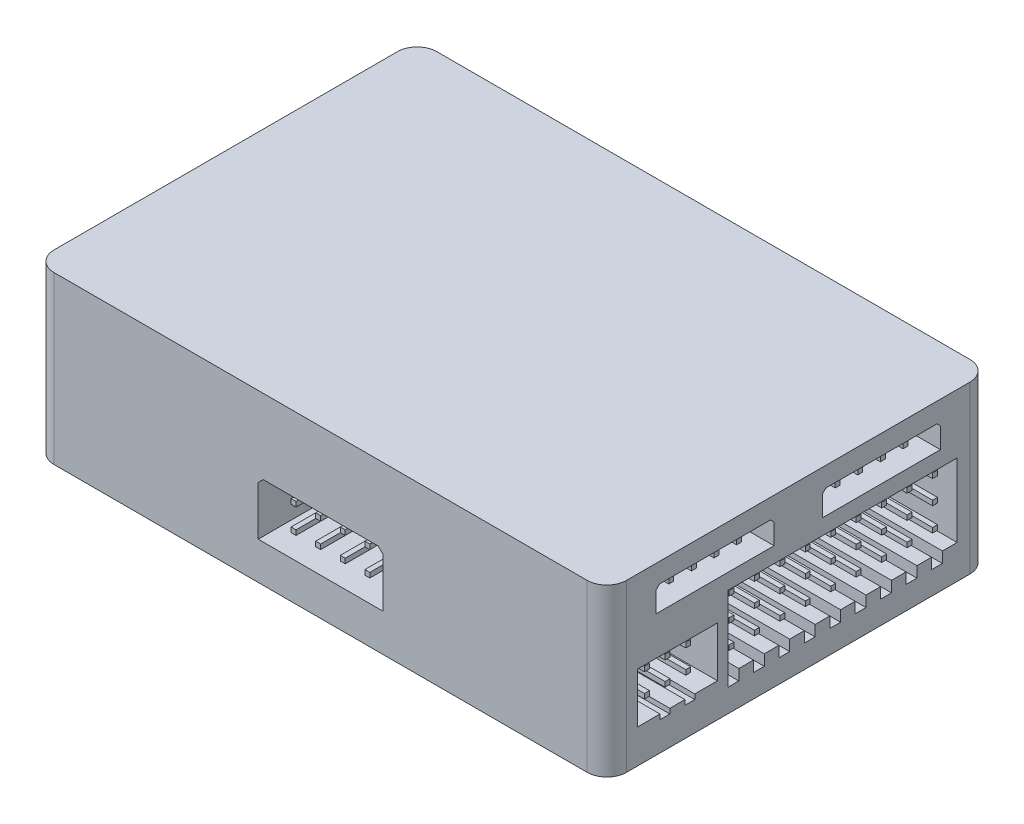
SolidWorks part; units mm, degrees
material "1060 合金"
ref_plane "前视基准面" through (0, 0, 0) normal (0, 0, 1) x (1, 0, 0)
ref_plane "上视基准面" through (0, 0, 0) normal (0, 1, 0) x (1, 0, 0)
ref_plane "右视基准面" through (0, 0, 0) normal (1, 0, 0) x (0, 0, -1)
other "质心 (COM)"
ref_plane "基准面4" through (0, 16.91, 0) normal (0, 1, 0) x (1, 0, 0)
sketch "草图1" plane through (0, 16.91, 0) normal (0, 1, 0) x (1, 0, 0)
  line L0 (29.105, -19.46) -> (29.105, 19.46)
  line L1 (29.105, 19.46) -> (-29.105, 19.46)
  line L2 (-29.105, 19.46) -> (-29.105, -19.46)
  line L3 (-29.105, -19.46) -> (29.105, -19.46)
extrude "凸台-拉伸1" add sketch "草图1" against normal blind 16.91
sketch "草图2" plane through (0, 0, 19.46) normal (0, 0, 1) x (1, 0, 0)
  line L0 (-6.35, 3.81) -> (6.35, 3.81)
  line L1 (6.35, 3.81) -> (6.35, 9.31)
  line L2 (6.35, 9.31) -> (-6.35, 9.31)
  line L3 (-6.35, 9.31) -> (-6.35, 3.81)
extrude "切除-拉伸1" cut sketch "草图2" against normal blind 10
sketch "草图3" plane through (0, 0, 9.46) normal (0, 0, 1) x (1, 0, 0)
  line L0 (-4, 8.06) -> (-3.5, 8.06)
  line L1 (-3.5, 8.06) -> (-3.5, 7.56)
  line L2 (-3.5, 7.56) -> (-4, 7.56)
  line L3 (-4, 7.56) -> (-4, 8.06)
extrude "凸台-拉伸2" add sketch "草图3" along normal blind 9
sketch "草图4" plane through (0, 0, 9.46) normal (0, 0, 1) x (1, 0, 0)
  line L0 (-4, 5.56) -> (-3.5, 5.56)
  line L1 (-3.5, 5.56) -> (-3.5, 5.06)
  line L2 (-3.5, 5.06) -> (-4, 5.06)
  line L3 (-4, 5.06) -> (-4, 5.56)
extrude "凸台-拉伸3" add sketch "草图4" along normal blind 9
sketch "草图5" plane through (0, 0, 9.46) normal (0, 0, 1) x (1, 0, 0)
  line L0 (-1.5, 8.06) -> (-1, 8.06)
  line L1 (-1, 8.06) -> (-1, 7.56)
  line L2 (-1, 7.56) -> (-1.5, 7.56)
  line L3 (-1.5, 7.56) -> (-1.5, 8.06)
extrude "凸台-拉伸4" add sketch "草图5" along normal blind 9
sketch "草图6" plane through (0, 0, 9.46) normal (0, 0, 1) x (1, 0, 0)
  line L0 (-1.5, 5.56) -> (-1, 5.56)
  line L1 (-1, 5.56) -> (-1, 5.06)
  line L2 (-1, 5.06) -> (-1.5, 5.06)
  line L3 (-1.5, 5.06) -> (-1.5, 5.56)
extrude "凸台-拉伸5" add sketch "草图6" along normal blind 9
sketch "草图7" plane through (0, 0, 9.46) normal (0, 0, 1) x (1, 0, 0)
  line L0 (1.5, 5.56) -> (1.5, 5.06)
  line L1 (1.5, 5.06) -> (1, 5.06)
  line L2 (1, 5.06) -> (1, 5.56)
  line L3 (1, 5.56) -> (1.5, 5.56)
extrude "凸台-拉伸6" add sketch "草图7" along normal blind 9
sketch "草图8" plane through (0, 0, 9.46) normal (0, 0, 1) x (1, 0, 0)
  line L0 (1.5, 8.06) -> (1.5, 7.56)
  line L1 (1.5, 7.56) -> (1, 7.56)
  line L2 (1, 7.56) -> (1, 8.06)
  line L3 (1, 8.06) -> (1.5, 8.06)
extrude "凸台-拉伸7" add sketch "草图8" along normal blind 9
sketch "草图9" plane through (0, 0, 9.46) normal (0, 0, 1) x (1, 0, 0)
  line L0 (4, 5.56) -> (4, 5.06)
  line L1 (4, 5.06) -> (3.5, 5.06)
  line L2 (3.5, 5.06) -> (3.5, 5.56)
  line L3 (3.5, 5.56) -> (4, 5.56)
extrude "凸台-拉伸8" add sketch "草图9" along normal blind 9
sketch "草图10" plane through (0, 0, 9.46) normal (0, 0, 1) x (1, 0, 0)
  line L0 (4, 8.06) -> (4, 7.56)
  line L1 (4, 7.56) -> (3.5, 7.56)
  line L2 (3.5, 7.56) -> (3.5, 8.06)
  line L3 (3.5, 8.06) -> (4, 8.06)
extrude "凸台-拉伸9" add sketch "草图10" along normal blind 9
sketch "草图11" plane through (29.105, 0, 0) normal (1, 0, 0) x (0, 0, -1)
  line L0 (13.56, 2.34) -> (14.66, 2.34)
  line L1 (14.66, 2.34) -> (14.66, 3.44)
  line L2 (14.66, 3.44) -> (16.16, 3.44)
  line L3 (16.16, 3.44) -> (16.16, 10.88)
  line L4 (16.16, 10.88) -> (-7.14, 10.88)
  line L5 (-7.14, 10.88) -> (-7.14, 2.34)
  line L6 (-7.14, 2.34) -> (-6.04, 2.34)
  line L7 (-6.04, 2.34) -> (-6.04, 3.44)
  line L8 (-6.04, 3.44) -> (-4.5525, 3.44)
  line L9 (-4.5525, 3.44) -> (-4.5525, 2.34)
  line L10 (-4.5525, 2.34) -> (-3.4525, 2.34)
  line L11 (-3.4525, 2.34) -> (-3.4525, 3.44)
  line L12 (-3.4525, 3.44) -> (-1.965, 3.44)
  line L13 (-1.965, 3.44) -> (-1.965, 2.34)
  line L14 (-1.965, 2.34) -> (-0.865, 2.34)
  line L15 (-0.865, 2.34) -> (-0.865, 3.44)
  line L16 (-0.865, 3.44) -> (0.6225, 3.44)
  line L17 (0.6225, 3.44) -> (0.6225, 2.34)
  line L18 (0.6225, 2.34) -> (1.7225, 2.34)
  line L19 (1.7225, 2.34) -> (1.7225, 3.44)
  line L20 (1.7225, 3.44) -> (3.21, 3.44)
  line L21 (3.21, 3.44) -> (3.21, 2.34)
  line L22 (3.21, 2.34) -> (4.31, 2.34)
  line L23 (4.31, 2.34) -> (4.31, 3.44)
  line L24 (4.31, 3.44) -> (5.7975, 3.44)
  line L25 (5.7975, 3.44) -> (5.7975, 2.34)
  line L26 (5.7975, 2.34) -> (6.8975, 2.34)
  line L27 (6.8975, 2.34) -> (6.8975, 3.44)
  line L28 (6.8975, 3.44) -> (8.385, 3.44)
  line L29 (8.385, 3.44) -> (8.385, 2.34)
  line L30 (8.385, 2.34) -> (9.485, 2.34)
  line L31 (9.485, 2.34) -> (9.485, 3.44)
  line L32 (9.485, 3.44) -> (10.9725, 3.44)
  line L33 (10.9725, 3.44) -> (10.9725, 2.34)
  line L34 (10.9725, 2.34) -> (12.0725, 2.34)
  line L35 (12.0725, 2.34) -> (12.0725, 3.44)
  line L36 (12.0725, 3.44) -> (13.56, 3.44)
  line L37 (13.56, 3.44) -> (13.56, 2.34)
extrude "切除-拉伸2" cut sketch "草图11" against normal blind 10
sketch "草图12" plane through (19.105, 0, 0) normal (1, 0, 0) x (0, 0, -1)
  line L0 (14.66, 7.41) -> (15.16, 7.41)
  line L1 (15.16, 7.41) -> (15.16, 6.91)
  line L2 (15.16, 6.91) -> (14.66, 6.91)
  line L3 (14.66, 6.91) -> (14.66, 7.41)
extrude "凸台-拉伸10" add sketch "草图12" along normal blind 9
sketch "草图13" plane through (19.105, 0, 0) normal (1, 0, 0) x (0, 0, -1)
  line L0 (12.0725, 5.01) -> (12.5725, 5.01)
  line L1 (12.5725, 5.01) -> (12.5725, 4.51)
  line L2 (12.5725, 4.51) -> (12.0725, 4.51)
  line L3 (12.0725, 4.51) -> (12.0725, 5.01)
extrude "凸台-拉伸11" add sketch "草图13" along normal blind 9
sketch "草图14" plane through (19.105, 0, 0) normal (1, 0, 0) x (0, 0, -1)
  line L0 (12.0725, 9.81) -> (12.5725, 9.81)
  line L1 (12.5725, 9.81) -> (12.5725, 9.31)
  line L2 (12.5725, 9.31) -> (12.0725, 9.31)
  line L3 (12.0725, 9.31) -> (12.0725, 9.81)
extrude "凸台-拉伸12" add sketch "草图14" along normal blind 9
sketch "草图15" plane through (19.105, 0, 0) normal (1, 0, 0) x (0, 0, -1)
  line L0 (9.485, 7.41) -> (9.985, 7.41)
  line L1 (9.985, 7.41) -> (9.985, 6.91)
  line L2 (9.985, 6.91) -> (9.485, 6.91)
  line L3 (9.485, 6.91) -> (9.485, 7.41)
extrude "凸台-拉伸13" add sketch "草图15" along normal blind 9
sketch "草图16" plane through (19.105, 0, 0) normal (1, 0, 0) x (0, 0, -1)
  line L0 (6.8975, 5.01) -> (7.3975, 5.01)
  line L1 (7.3975, 5.01) -> (7.3975, 4.51)
  line L2 (7.3975, 4.51) -> (6.8975, 4.51)
  line L3 (6.8975, 4.51) -> (6.8975, 5.01)
extrude "凸台-拉伸14" add sketch "草图16" along normal blind 9
sketch "草图17" plane through (19.105, 0, 0) normal (1, 0, 0) x (0, 0, -1)
  line L0 (6.8975, 9.81) -> (7.3975, 9.81)
  line L1 (7.3975, 9.81) -> (7.3975, 9.31)
  line L2 (7.3975, 9.31) -> (6.8975, 9.31)
  line L3 (6.8975, 9.31) -> (6.8975, 9.81)
extrude "凸台-拉伸15" add sketch "草图17" along normal blind 9
sketch "草图18" plane through (19.105, 0, 0) normal (1, 0, 0) x (0, 0, -1)
  line L0 (4.31, 7.41) -> (4.81, 7.41)
  line L1 (4.81, 7.41) -> (4.81, 6.91)
  line L2 (4.81, 6.91) -> (4.31, 6.91)
  line L3 (4.31, 6.91) -> (4.31, 7.41)
extrude "凸台-拉伸16" add sketch "草图18" along normal blind 9
sketch "草图19" plane through (19.105, 0, 0) normal (1, 0, 0) x (0, 0, -1)
  line L0 (1.7225, 5.01) -> (2.2225, 5.01)
  line L1 (2.2225, 5.01) -> (2.2225, 4.51)
  line L2 (2.2225, 4.51) -> (1.7225, 4.51)
  line L3 (1.7225, 4.51) -> (1.7225, 5.01)
extrude "凸台-拉伸17" add sketch "草图19" along normal blind 9
sketch "草图20" plane through (19.105, 0, 0) normal (1, 0, 0) x (0, 0, -1)
  line L0 (1.7225, 9.81) -> (2.2225, 9.81)
  line L1 (2.2225, 9.81) -> (2.2225, 9.31)
  line L2 (2.2225, 9.31) -> (1.7225, 9.31)
  line L3 (1.7225, 9.31) -> (1.7225, 9.81)
extrude "凸台-拉伸18" add sketch "草图20" along normal blind 9
sketch "草图21" plane through (19.105, 0, 0) normal (1, 0, 0) x (0, 0, -1)
  line L0 (-0.865, 7.41) -> (-0.365, 7.41)
  line L1 (-0.365, 7.41) -> (-0.365, 6.91)
  line L2 (-0.365, 6.91) -> (-0.865, 6.91)
  line L3 (-0.865, 6.91) -> (-0.865, 7.41)
extrude "凸台-拉伸19" add sketch "草图21" along normal blind 9
sketch "草图22" plane through (19.105, 0, 0) normal (1, 0, 0) x (0, 0, -1)
  line L0 (-3.4525, 5.01) -> (-2.9525, 5.01)
  line L1 (-2.9525, 5.01) -> (-2.9525, 4.51)
  line L2 (-2.9525, 4.51) -> (-3.4525, 4.51)
  line L3 (-3.4525, 4.51) -> (-3.4525, 5.01)
extrude "凸台-拉伸20" add sketch "草图22" along normal blind 9
sketch "草图23" plane through (19.105, 0, 0) normal (1, 0, 0) x (0, 0, -1)
  line L0 (-3.4525, 9.81) -> (-2.9525, 9.81)
  line L1 (-2.9525, 9.81) -> (-2.9525, 9.31)
  line L2 (-2.9525, 9.31) -> (-3.4525, 9.31)
  line L3 (-3.4525, 9.31) -> (-3.4525, 9.81)
extrude "凸台-拉伸21" add sketch "草图23" along normal blind 9
sketch "草图24" plane through (19.105, 0, 0) normal (1, 0, 0) x (0, 0, -1)
  line L0 (-6.04, 7.41) -> (-5.54, 7.41)
  line L1 (-5.54, 7.41) -> (-5.54, 6.91)
  line L2 (-5.54, 6.91) -> (-6.04, 6.91)
  line L3 (-6.04, 6.91) -> (-6.04, 7.41)
extrude "凸台-拉伸22" add sketch "草图24" along normal blind 9
sketch "草图25" plane through (19.105, 0, 0) normal (1, 0, 0) x (0, 0, -1)
  line L0 (-6.04, 9.81) -> (-5.54, 9.81)
  line L1 (-5.54, 9.81) -> (-5.54, 9.31)
  line L2 (-5.54, 9.31) -> (-6.04, 9.31)
  line L3 (-6.04, 9.31) -> (-6.04, 9.81)
extrude "凸台-拉伸23" add sketch "草图25" along normal blind 9
sketch "草图26" plane through (19.105, 0, 0) normal (1, 0, 0) x (0, 0, -1)
  line L0 (-6.04, 5.01) -> (-5.54, 5.01)
  line L1 (-5.54, 5.01) -> (-5.54, 4.51)
  line L2 (-5.54, 4.51) -> (-6.04, 4.51)
  line L3 (-6.04, 4.51) -> (-6.04, 5.01)
extrude "凸台-拉伸24" add sketch "草图26" along normal blind 9
sketch "草图27" plane through (19.105, 0, 0) normal (1, 0, 0) x (0, 0, -1)
  line L0 (-3.4525, 7.41) -> (-2.9525, 7.41)
  line L1 (-2.9525, 7.41) -> (-2.9525, 6.91)
  line L2 (-2.9525, 6.91) -> (-3.4525, 6.91)
  line L3 (-3.4525, 6.91) -> (-3.4525, 7.41)
extrude "凸台-拉伸25" add sketch "草图27" along normal blind 9
sketch "草图28" plane through (19.105, 0, 0) normal (1, 0, 0) x (0, 0, -1)
  line L0 (-0.865, 9.81) -> (-0.365, 9.81)
  line L1 (-0.365, 9.81) -> (-0.365, 9.31)
  line L2 (-0.365, 9.31) -> (-0.865, 9.31)
  line L3 (-0.865, 9.31) -> (-0.865, 9.81)
extrude "凸台-拉伸26" add sketch "草图28" along normal blind 9
sketch "草图29" plane through (19.105, 0, 0) normal (1, 0, 0) x (0, 0, -1)
  line L0 (-0.865, 5.01) -> (-0.365, 5.01)
  line L1 (-0.365, 5.01) -> (-0.365, 4.51)
  line L2 (-0.365, 4.51) -> (-0.865, 4.51)
  line L3 (-0.865, 4.51) -> (-0.865, 5.01)
extrude "凸台-拉伸27" add sketch "草图29" along normal blind 9
sketch "草图30" plane through (19.105, 0, 0) normal (1, 0, 0) x (0, 0, -1)
  line L0 (1.7225, 7.41) -> (2.2225, 7.41)
  line L1 (2.2225, 7.41) -> (2.2225, 6.91)
  line L2 (2.2225, 6.91) -> (1.7225, 6.91)
  line L3 (1.7225, 6.91) -> (1.7225, 7.41)
extrude "凸台-拉伸28" add sketch "草图30" along normal blind 9
sketch "草图31" plane through (19.105, 0, 0) normal (1, 0, 0) x (0, 0, -1)
  line L0 (4.31, 9.81) -> (4.81, 9.81)
  line L1 (4.81, 9.81) -> (4.81, 9.31)
  line L2 (4.81, 9.31) -> (4.31, 9.31)
  line L3 (4.31, 9.31) -> (4.31, 9.81)
extrude "凸台-拉伸29" add sketch "草图31" along normal blind 9
sketch "草图32" plane through (19.105, 0, 0) normal (1, 0, 0) x (0, 0, -1)
  line L0 (4.31, 5.01) -> (4.81, 5.01)
  line L1 (4.81, 5.01) -> (4.81, 4.51)
  line L2 (4.81, 4.51) -> (4.31, 4.51)
  line L3 (4.31, 4.51) -> (4.31, 5.01)
extrude "凸台-拉伸30" add sketch "草图32" along normal blind 9
sketch "草图33" plane through (19.105, 0, 0) normal (1, 0, 0) x (0, 0, -1)
  line L0 (6.8975, 7.41) -> (7.3975, 7.41)
  line L1 (7.3975, 7.41) -> (7.3975, 6.91)
  line L2 (7.3975, 6.91) -> (6.8975, 6.91)
  line L3 (6.8975, 6.91) -> (6.8975, 7.41)
extrude "凸台-拉伸31" add sketch "草图33" along normal blind 9
sketch "草图34" plane through (19.105, 0, 0) normal (1, 0, 0) x (0, 0, -1)
  line L0 (9.485, 9.81) -> (9.985, 9.81)
  line L1 (9.985, 9.81) -> (9.985, 9.31)
  line L2 (9.985, 9.31) -> (9.485, 9.31)
  line L3 (9.485, 9.31) -> (9.485, 9.81)
extrude "凸台-拉伸32" add sketch "草图34" along normal blind 9
sketch "草图35" plane through (19.105, 0, 0) normal (1, 0, 0) x (0, 0, -1)
  line L0 (9.485, 5.01) -> (9.985, 5.01)
  line L1 (9.985, 5.01) -> (9.985, 4.51)
  line L2 (9.985, 4.51) -> (9.485, 4.51)
  line L3 (9.485, 4.51) -> (9.485, 5.01)
extrude "凸台-拉伸33" add sketch "草图35" along normal blind 9
sketch "草图36" plane through (19.105, 0, 0) normal (1, 0, 0) x (0, 0, -1)
  line L0 (12.0725, 7.41) -> (12.5725, 7.41)
  line L1 (12.5725, 7.41) -> (12.5725, 6.91)
  line L2 (12.5725, 6.91) -> (12.0725, 6.91)
  line L3 (12.0725, 6.91) -> (12.0725, 7.41)
extrude "凸台-拉伸34" add sketch "草图36" along normal blind 9
sketch "草图37" plane through (19.105, 0, 0) normal (1, 0, 0) x (0, 0, -1)
  line L0 (14.66, 9.81) -> (15.16, 9.81)
  line L1 (15.16, 9.81) -> (15.16, 9.31)
  line L2 (15.16, 9.31) -> (14.66, 9.31)
  line L3 (14.66, 9.31) -> (14.66, 9.81)
extrude "凸台-拉伸35" add sketch "草图37" along normal blind 9
sketch "草图38" plane through (19.105, 0, 0) normal (1, 0, 0) x (0, 0, -1)
  line L0 (14.66, 5.01) -> (15.16, 5.01)
  line L1 (15.16, 5.01) -> (15.16, 4.51)
  line L2 (15.16, 4.51) -> (14.66, 4.51)
  line L3 (14.66, 4.51) -> (14.66, 5.01)
extrude "凸台-拉伸36" add sketch "草图38" along normal blind 9
sketch "草图39" plane through (29.105, 0, 0) normal (1, 0, 0) x (0, 0, -1)
  line L0 (-14.46, 12.46) -> (-2.46, 12.46)
  line L1 (-2.46, 12.46) -> (-2.46, 14.91)
  line L2 (-2.46, 14.91) -> (-14.46, 14.91)
  line L3 (-14.46, 14.91) -> (-14.46, 12.46)
extrude "切除-拉伸3" cut sketch "草图39" against normal blind 10
sketch "草图40" plane through (19.105, 0, 0) normal (1, 0, 0) x (0, 0, -1)
  line L0 (-7.06, 13.935) -> (-7.06, 13.435)
  line L1 (-7.06, 13.435) -> (-7.56, 13.435)
  line L2 (-7.56, 13.435) -> (-7.56, 13.935)
  line L3 (-7.56, 13.935) -> (-7.06, 13.935)
extrude "凸台-拉伸37" add sketch "草图40" along normal blind 9
sketch "草图41" plane through (19.105, 0, 0) normal (1, 0, 0) x (0, 0, -1)
  line L0 (-12.16, 13.935) -> (-11.66, 13.935)
  line L1 (-11.66, 13.935) -> (-11.66, 13.435)
  line L2 (-11.66, 13.435) -> (-12.16, 13.435)
  line L3 (-12.16, 13.435) -> (-12.16, 13.935)
extrude "凸台-拉伸38" add sketch "草图41" along normal blind 9
sketch "草图42" plane through (19.105, 0, 0) normal (1, 0, 0) x (0, 0, -1)
  line L0 (-9.86, 13.935) -> (-9.36, 13.935)
  line L1 (-9.36, 13.935) -> (-9.36, 13.435)
  line L2 (-9.36, 13.435) -> (-9.86, 13.435)
  line L3 (-9.86, 13.435) -> (-9.86, 13.935)
extrude "凸台-拉伸39" add sketch "草图42" along normal blind 9
sketch "草图43" plane through (19.105, 0, 0) normal (1, 0, 0) x (0, 0, -1)
  line L0 (-4.76, 13.935) -> (-4.76, 13.435)
  line L1 (-4.76, 13.435) -> (-5.26, 13.435)
  line L2 (-5.26, 13.435) -> (-5.26, 13.935)
  line L3 (-5.26, 13.935) -> (-4.76, 13.935)
extrude "凸台-拉伸40" add sketch "草图43" along normal blind 9
sketch "草图44" plane through (29.105, 0, 0) normal (1, 0, 0) x (0, 0, -1)
  line L0 (-11.515, 2.94) -> (-10.515, 2.94)
  line L1 (-10.515, 2.94) -> (-10.515, 3.44)
  line L2 (-10.515, 3.44) -> (-8.21, 3.44)
  line L3 (-8.21, 3.44) -> (-8.21, 8.54)
  line L4 (-8.21, 8.54) -> (-16.36, 8.54)
  line L5 (-16.36, 8.54) -> (-16.36, 3.44)
  line L6 (-16.36, 3.44) -> (-14.055, 3.44)
  line L7 (-14.055, 3.44) -> (-14.055, 2.94)
  line L8 (-14.055, 2.94) -> (-13.055, 2.94)
  line L9 (-13.055, 2.94) -> (-13.055, 3.44)
  line L10 (-13.055, 3.44) -> (-11.515, 3.44)
  line L11 (-11.515, 3.44) -> (-11.515, 2.94)
extrude "切除-拉伸4" cut sketch "草图44" against normal blind 10
sketch "草图45" plane through (19.105, 0, 0) normal (1, 0, 0) x (0, 0, -1)
  line L0 (-14.135, 6.94) -> (-14.635, 6.94)
  line L1 (-14.635, 6.94) -> (-14.635, 7.44)
  line L2 (-14.635, 7.44) -> (-14.135, 7.44)
  line L3 (-14.135, 7.44) -> (-14.135, 6.94)
extrude "凸台-拉伸41" add sketch "草图45" along normal blind 9
sketch "草图46" plane through (19.105, 0, 0) normal (1, 0, 0) x (0, 0, -1)
  line L0 (-9.935, 6.94) -> (-10.435, 6.94)
  line L1 (-10.435, 6.94) -> (-10.435, 7.44)
  line L2 (-10.435, 7.44) -> (-9.935, 7.44)
  line L3 (-9.935, 7.44) -> (-9.935, 6.94)
extrude "凸台-拉伸42" add sketch "草图46" along normal blind 9
sketch "草图47" plane through (19.105, 0, 0) normal (1, 0, 0) x (0, 0, -1)
  line L0 (-12.035, 6.94) -> (-12.535, 6.94)
  line L1 (-12.535, 6.94) -> (-12.535, 7.44)
  line L2 (-12.535, 7.44) -> (-12.035, 7.44)
  line L3 (-12.035, 7.44) -> (-12.035, 6.94)
extrude "凸台-拉伸43" add sketch "草图47" along normal blind 9
sketch "草图48" plane through (19.105, 0, 0) normal (1, 0, 0) x (0, 0, -1)
  line L0 (-12.035, 5.04) -> (-12.035, 4.54)
  line L1 (-12.035, 4.54) -> (-12.535, 4.54)
  line L2 (-12.535, 4.54) -> (-12.535, 5.04)
  line L3 (-12.535, 5.04) -> (-12.035, 5.04)
extrude "凸台-拉伸44" add sketch "草图48" along normal blind 9
sketch "草图49" plane through (19.105, 0, 0) normal (1, 0, 0) x (0, 0, -1)
  line L0 (-9.935, 5.04) -> (-9.935, 4.54)
  line L1 (-9.935, 4.54) -> (-10.435, 4.54)
  line L2 (-10.435, 4.54) -> (-10.435, 5.04)
  line L3 (-10.435, 5.04) -> (-9.935, 5.04)
extrude "凸台-拉伸45" add sketch "草图49" along normal blind 9
sketch "草图50" plane through (19.105, 0, 0) normal (1, 0, 0) x (0, 0, -1)
  line L0 (-14.135, 5.04) -> (-14.135, 4.54)
  line L1 (-14.135, 4.54) -> (-14.635, 4.54)
  line L2 (-14.635, 4.54) -> (-14.635, 5.04)
  line L3 (-14.635, 5.04) -> (-14.135, 5.04)
extrude "凸台-拉伸46" add sketch "草图50" along normal blind 9
sketch "草图51" plane through (29.105, 0, 0) normal (1, 0, 0) x (0, 0, -1)
  line L0 (2.46, 12.46) -> (14.46, 12.46)
  line L1 (14.46, 12.46) -> (14.46, 14.91)
  line L2 (14.46, 14.91) -> (2.46, 14.91)
  line L3 (2.46, 14.91) -> (2.46, 12.46)
extrude "切除-拉伸5" cut sketch "草图51" against normal blind 10
sketch "草图52" plane through (19.105, 0, 0) normal (1, 0, 0) x (0, 0, -1)
  line L0 (9.86, 13.935) -> (9.86, 13.435)
  line L1 (9.86, 13.435) -> (9.36, 13.435)
  line L2 (9.36, 13.435) -> (9.36, 13.935)
  line L3 (9.36, 13.935) -> (9.86, 13.935)
extrude "凸台-拉伸47" add sketch "草图52" along normal blind 9
sketch "草图53" plane through (19.105, 0, 0) normal (1, 0, 0) x (0, 0, -1)
  line L0 (4.76, 13.935) -> (5.26, 13.935)
  line L1 (5.26, 13.935) -> (5.26, 13.435)
  line L2 (5.26, 13.435) -> (4.76, 13.435)
  line L3 (4.76, 13.435) -> (4.76, 13.935)
extrude "凸台-拉伸48" add sketch "草图53" along normal blind 9
sketch "草图54" plane through (19.105, 0, 0) normal (1, 0, 0) x (0, 0, -1)
  line L0 (7.06, 13.935) -> (7.56, 13.935)
  line L1 (7.56, 13.935) -> (7.56, 13.435)
  line L2 (7.56, 13.435) -> (7.06, 13.435)
  line L3 (7.06, 13.435) -> (7.06, 13.935)
extrude "凸台-拉伸49" add sketch "草图54" along normal blind 9
sketch "草图55" plane through (19.105, 0, 0) normal (1, 0, 0) x (0, 0, -1)
  line L0 (12.16, 13.935) -> (12.16, 13.435)
  line L1 (12.16, 13.435) -> (11.66, 13.435)
  line L2 (11.66, 13.435) -> (11.66, 13.935)
  line L3 (11.66, 13.935) -> (12.16, 13.935)
extrude "凸台-拉伸50" add sketch "草图55" along normal blind 9
sketch "草图56" plane through (-29.105, 0, 0) normal (-1, 0, 0) x (0, 0, 1)
  line L0 (5.64, 3.44) -> (7.14, 3.44)
  line L1 (7.14, 3.44) -> (7.14, 10.88)
  line L2 (7.14, 10.88) -> (-16.16, 10.88)
  line L3 (-16.16, 10.88) -> (-16.16, 2.34)
  line L4 (-16.16, 2.34) -> (-15.06, 2.34)
  line L5 (-15.06, 2.34) -> (-15.06, 3.44)
  line L6 (-15.06, 3.44) -> (-13.5725, 3.44)
  line L7 (-13.5725, 3.44) -> (-13.5725, 2.34)
  line L8 (-13.5725, 2.34) -> (-12.4725, 2.34)
  line L9 (-12.4725, 2.34) -> (-12.4725, 3.44)
  line L10 (-12.4725, 3.44) -> (-10.985, 3.44)
  line L11 (-10.985, 3.44) -> (-10.985, 2.34)
  line L12 (-10.985, 2.34) -> (-9.885, 2.34)
  line L13 (-9.885, 2.34) -> (-9.885, 3.44)
  line L14 (-9.885, 3.44) -> (-8.3975, 3.44)
  line L15 (-8.3975, 3.44) -> (-8.3975, 2.34)
  line L16 (-8.3975, 2.34) -> (-7.2975, 2.34)
  line L17 (-7.2975, 2.34) -> (-7.2975, 3.44)
  line L18 (-7.2975, 3.44) -> (-5.81, 3.44)
  line L19 (-5.81, 3.44) -> (-5.81, 2.34)
  line L20 (-5.81, 2.34) -> (-4.71, 2.34)
  line L21 (-4.71, 2.34) -> (-4.71, 3.44)
  line L22 (-4.71, 3.44) -> (-3.2225, 3.44)
  line L23 (-3.2225, 3.44) -> (-3.2225, 2.34)
  line L24 (-3.2225, 2.34) -> (-2.1225, 2.34)
  line L25 (-2.1225, 2.34) -> (-2.1225, 3.44)
  line L26 (-2.1225, 3.44) -> (-0.635, 3.44)
  line L27 (-0.635, 3.44) -> (-0.635, 2.34)
  line L28 (-0.635, 2.34) -> (0.465, 2.34)
  line L29 (0.465, 2.34) -> (0.465, 3.44)
  line L30 (0.465, 3.44) -> (1.9525, 3.44)
  line L31 (1.9525, 3.44) -> (1.9525, 2.34)
  line L32 (1.9525, 2.34) -> (3.0525, 2.34)
  line L33 (3.0525, 2.34) -> (3.0525, 3.44)
  line L34 (3.0525, 3.44) -> (4.54, 3.44)
  line L35 (4.54, 3.44) -> (4.54, 2.34)
  line L36 (4.54, 2.34) -> (5.64, 2.34)
  line L37 (5.64, 2.34) -> (5.64, 3.44)
extrude "切除-拉伸6" cut sketch "草图56" against normal blind 10
sketch "草图57" plane through (-19.105, 0, 0) normal (-1, 0, 0) x (0, 0, 1)
  line L0 (6.04, 9.31) -> (5.54, 9.31)
  line L1 (5.54, 9.31) -> (5.54, 9.81)
  line L2 (5.54, 9.81) -> (6.04, 9.81)
  line L3 (6.04, 9.81) -> (6.04, 9.31)
extrude "凸台-拉伸51" add sketch "草图57" along normal blind 9
sketch "草图58" plane through (-19.105, 0, 0) normal (-1, 0, 0) x (0, 0, 1)
  line L0 (6.04, 6.91) -> (5.54, 6.91)
  line L1 (5.54, 6.91) -> (5.54, 7.41)
  line L2 (5.54, 7.41) -> (6.04, 7.41)
  line L3 (6.04, 7.41) -> (6.04, 6.91)
extrude "凸台-拉伸52" add sketch "草图58" along normal blind 9
sketch "草图59" plane through (-19.105, 0, 0) normal (-1, 0, 0) x (0, 0, 1)
  line L0 (6.04, 4.51) -> (5.54, 4.51)
  line L1 (5.54, 4.51) -> (5.54, 5.01)
  line L2 (5.54, 5.01) -> (6.04, 5.01)
  line L3 (6.04, 5.01) -> (6.04, 4.51)
extrude "凸台-拉伸53" add sketch "草图59" along normal blind 9
sketch "草图60" plane through (-19.105, 0, 0) normal (-1, 0, 0) x (0, 0, 1)
  line L0 (3.4525, 9.31) -> (2.9525, 9.31)
  line L1 (2.9525, 9.31) -> (2.9525, 9.81)
  line L2 (2.9525, 9.81) -> (3.4525, 9.81)
  line L3 (3.4525, 9.81) -> (3.4525, 9.31)
extrude "凸台-拉伸54" add sketch "草图60" along normal blind 9
sketch "草图61" plane through (-19.105, 0, 0) normal (-1, 0, 0) x (0, 0, 1)
  line L0 (3.4525, 6.91) -> (2.9525, 6.91)
  line L1 (2.9525, 6.91) -> (2.9525, 7.41)
  line L2 (2.9525, 7.41) -> (3.4525, 7.41)
  line L3 (3.4525, 7.41) -> (3.4525, 6.91)
extrude "凸台-拉伸55" add sketch "草图61" along normal blind 9
sketch "草图62" plane through (-19.105, 0, 0) normal (-1, 0, 0) x (0, 0, 1)
  line L0 (3.4525, 4.51) -> (2.9525, 4.51)
  line L1 (2.9525, 4.51) -> (2.9525, 5.01)
  line L2 (2.9525, 5.01) -> (3.4525, 5.01)
  line L3 (3.4525, 5.01) -> (3.4525, 4.51)
extrude "凸台-拉伸56" add sketch "草图62" along normal blind 9
sketch "草图63" plane through (-19.105, 0, 0) normal (-1, 0, 0) x (0, 0, 1)
  line L0 (0.865, 9.31) -> (0.365, 9.31)
  line L1 (0.365, 9.31) -> (0.365, 9.81)
  line L2 (0.365, 9.81) -> (0.865, 9.81)
  line L3 (0.865, 9.81) -> (0.865, 9.31)
extrude "凸台-拉伸57" add sketch "草图63" along normal blind 9
sketch "草图64" plane through (-19.105, 0, 0) normal (-1, 0, 0) x (0, 0, 1)
  line L0 (0.865, 6.91) -> (0.365, 6.91)
  line L1 (0.365, 6.91) -> (0.365, 7.41)
  line L2 (0.365, 7.41) -> (0.865, 7.41)
  line L3 (0.865, 7.41) -> (0.865, 6.91)
extrude "凸台-拉伸58" add sketch "草图64" along normal blind 9
sketch "草图65" plane through (-19.105, 0, 0) normal (-1, 0, 0) x (0, 0, 1)
  line L0 (0.865, 4.51) -> (0.365, 4.51)
  line L1 (0.365, 4.51) -> (0.365, 5.01)
  line L2 (0.365, 5.01) -> (0.865, 5.01)
  line L3 (0.865, 5.01) -> (0.865, 4.51)
extrude "凸台-拉伸59" add sketch "草图65" along normal blind 9
sketch "草图66" plane through (-19.105, 0, 0) normal (-1, 0, 0) x (0, 0, 1)
  line L0 (-1.7225, 9.31) -> (-2.2225, 9.31)
  line L1 (-2.2225, 9.31) -> (-2.2225, 9.81)
  line L2 (-2.2225, 9.81) -> (-1.7225, 9.81)
  line L3 (-1.7225, 9.81) -> (-1.7225, 9.31)
extrude "凸台-拉伸60" add sketch "草图66" along normal blind 9
sketch "草图67" plane through (-19.105, 0, 0) normal (-1, 0, 0) x (0, 0, 1)
  line L0 (-1.7225, 6.91) -> (-2.2225, 6.91)
  line L1 (-2.2225, 6.91) -> (-2.2225, 7.41)
  line L2 (-2.2225, 7.41) -> (-1.7225, 7.41)
  line L3 (-1.7225, 7.41) -> (-1.7225, 6.91)
extrude "凸台-拉伸61" add sketch "草图67" along normal blind 9
sketch "草图68" plane through (-19.105, 0, 0) normal (-1, 0, 0) x (0, 0, 1)
  line L0 (-1.7225, 4.51) -> (-2.2225, 4.51)
  line L1 (-2.2225, 4.51) -> (-2.2225, 5.01)
  line L2 (-2.2225, 5.01) -> (-1.7225, 5.01)
  line L3 (-1.7225, 5.01) -> (-1.7225, 4.51)
extrude "凸台-拉伸62" add sketch "草图68" along normal blind 9
sketch "草图69" plane through (-19.105, 0, 0) normal (-1, 0, 0) x (0, 0, 1)
  line L0 (-4.31, 9.31) -> (-4.81, 9.31)
  line L1 (-4.81, 9.31) -> (-4.81, 9.81)
  line L2 (-4.81, 9.81) -> (-4.31, 9.81)
  line L3 (-4.31, 9.81) -> (-4.31, 9.31)
extrude "凸台-拉伸63" add sketch "草图69" along normal blind 9
sketch "草图70" plane through (-19.105, 0, 0) normal (-1, 0, 0) x (0, 0, 1)
  line L0 (-4.31, 6.91) -> (-4.81, 6.91)
  line L1 (-4.81, 6.91) -> (-4.81, 7.41)
  line L2 (-4.81, 7.41) -> (-4.31, 7.41)
  line L3 (-4.31, 7.41) -> (-4.31, 6.91)
extrude "凸台-拉伸64" add sketch "草图70" along normal blind 9
sketch "草图71" plane through (-19.105, 0, 0) normal (-1, 0, 0) x (0, 0, 1)
  line L0 (-4.31, 4.51) -> (-4.81, 4.51)
  line L1 (-4.81, 4.51) -> (-4.81, 5.01)
  line L2 (-4.81, 5.01) -> (-4.31, 5.01)
  line L3 (-4.31, 5.01) -> (-4.31, 4.51)
extrude "凸台-拉伸65" add sketch "草图71" along normal blind 9
sketch "草图72" plane through (-19.105, 0, 0) normal (-1, 0, 0) x (0, 0, 1)
  line L0 (-6.8975, 9.31) -> (-7.3975, 9.31)
  line L1 (-7.3975, 9.31) -> (-7.3975, 9.81)
  line L2 (-7.3975, 9.81) -> (-6.8975, 9.81)
  line L3 (-6.8975, 9.81) -> (-6.8975, 9.31)
extrude "凸台-拉伸66" add sketch "草图72" along normal blind 9
sketch "草图73" plane through (-19.105, 0, 0) normal (-1, 0, 0) x (0, 0, 1)
  line L0 (-6.8975, 6.91) -> (-7.3975, 6.91)
  line L1 (-7.3975, 6.91) -> (-7.3975, 7.41)
  line L2 (-7.3975, 7.41) -> (-6.8975, 7.41)
  line L3 (-6.8975, 7.41) -> (-6.8975, 6.91)
extrude "凸台-拉伸67" add sketch "草图73" along normal blind 9
sketch "草图74" plane through (-19.105, 0, 0) normal (-1, 0, 0) x (0, 0, 1)
  line L0 (-6.8975, 4.51) -> (-7.3975, 4.51)
  line L1 (-7.3975, 4.51) -> (-7.3975, 5.01)
  line L2 (-7.3975, 5.01) -> (-6.8975, 5.01)
  line L3 (-6.8975, 5.01) -> (-6.8975, 4.51)
extrude "凸台-拉伸68" add sketch "草图74" along normal blind 9
sketch "草图75" plane through (-19.105, 0, 0) normal (-1, 0, 0) x (0, 0, 1)
  line L0 (-9.485, 9.31) -> (-9.985, 9.31)
  line L1 (-9.985, 9.31) -> (-9.985, 9.81)
  line L2 (-9.985, 9.81) -> (-9.485, 9.81)
  line L3 (-9.485, 9.81) -> (-9.485, 9.31)
extrude "凸台-拉伸69" add sketch "草图75" along normal blind 9
sketch "草图76" plane through (-19.105, 0, 0) normal (-1, 0, 0) x (0, 0, 1)
  line L0 (-9.485, 6.91) -> (-9.985, 6.91)
  line L1 (-9.985, 6.91) -> (-9.985, 7.41)
  line L2 (-9.985, 7.41) -> (-9.485, 7.41)
  line L3 (-9.485, 7.41) -> (-9.485, 6.91)
extrude "凸台-拉伸70" add sketch "草图76" along normal blind 9
sketch "草图77" plane through (-19.105, 0, 0) normal (-1, 0, 0) x (0, 0, 1)
  line L0 (-9.485, 4.51) -> (-9.985, 4.51)
  line L1 (-9.985, 4.51) -> (-9.985, 5.01)
  line L2 (-9.985, 5.01) -> (-9.485, 5.01)
  line L3 (-9.485, 5.01) -> (-9.485, 4.51)
extrude "凸台-拉伸71" add sketch "草图77" along normal blind 9
sketch "草图78" plane through (-19.105, 0, 0) normal (-1, 0, 0) x (0, 0, 1)
  line L0 (-12.0725, 9.31) -> (-12.5725, 9.31)
  line L1 (-12.5725, 9.31) -> (-12.5725, 9.81)
  line L2 (-12.5725, 9.81) -> (-12.0725, 9.81)
  line L3 (-12.0725, 9.81) -> (-12.0725, 9.31)
extrude "凸台-拉伸72" add sketch "草图78" along normal blind 9
sketch "草图79" plane through (-19.105, 0, 0) normal (-1, 0, 0) x (0, 0, 1)
  line L0 (-12.0725, 6.91) -> (-12.5725, 6.91)
  line L1 (-12.5725, 6.91) -> (-12.5725, 7.41)
  line L2 (-12.5725, 7.41) -> (-12.0725, 7.41)
  line L3 (-12.0725, 7.41) -> (-12.0725, 6.91)
extrude "凸台-拉伸73" add sketch "草图79" along normal blind 9
sketch "草图80" plane through (-19.105, 0, 0) normal (-1, 0, 0) x (0, 0, 1)
  line L0 (-12.0725, 4.51) -> (-12.5725, 4.51)
  line L1 (-12.5725, 4.51) -> (-12.5725, 5.01)
  line L2 (-12.5725, 5.01) -> (-12.0725, 5.01)
  line L3 (-12.0725, 5.01) -> (-12.0725, 4.51)
extrude "凸台-拉伸74" add sketch "草图80" along normal blind 9
sketch "草图81" plane through (-19.105, 0, 0) normal (-1, 0, 0) x (0, 0, 1)
  line L0 (-14.66, 9.31) -> (-15.16, 9.31)
  line L1 (-15.16, 9.31) -> (-15.16, 9.81)
  line L2 (-15.16, 9.81) -> (-14.66, 9.81)
  line L3 (-14.66, 9.81) -> (-14.66, 9.31)
extrude "凸台-拉伸75" add sketch "草图81" along normal blind 9
sketch "草图82" plane through (-19.105, 0, 0) normal (-1, 0, 0) x (0, 0, 1)
  line L0 (-14.66, 6.91) -> (-15.16, 6.91)
  line L1 (-15.16, 6.91) -> (-15.16, 7.41)
  line L2 (-15.16, 7.41) -> (-14.66, 7.41)
  line L3 (-14.66, 7.41) -> (-14.66, 6.91)
extrude "凸台-拉伸76" add sketch "草图82" along normal blind 9
sketch "草图83" plane through (-19.105, 0, 0) normal (-1, 0, 0) x (0, 0, 1)
  line L0 (-14.66, 4.51) -> (-15.16, 4.51)
  line L1 (-15.16, 4.51) -> (-15.16, 5.01)
  line L2 (-15.16, 5.01) -> (-14.66, 5.01)
  line L3 (-14.66, 5.01) -> (-14.66, 4.51)
extrude "凸台-拉伸77" add sketch "草图83" along normal blind 9
sketch "草图84" plane through (-29.105, 0, 0) normal (-1, 0, 0) x (0, 0, 1)
  line L0 (-14.46, 12.46) -> (-2.46, 12.46)
  line L1 (-2.46, 12.46) -> (-2.46, 14.91)
  line L2 (-2.46, 14.91) -> (-14.46, 14.91)
  line L3 (-14.46, 14.91) -> (-14.46, 12.46)
extrude "切除-拉伸7" cut sketch "草图84" against normal blind 10
sketch "草图85" plane through (-19.105, 0, 0) normal (-1, 0, 0) x (0, 0, 1)
  line L0 (-12.16, 13.435) -> (-12.16, 13.935)
  line L1 (-12.16, 13.935) -> (-11.66, 13.935)
  line L2 (-11.66, 13.935) -> (-11.66, 13.435)
  line L3 (-11.66, 13.435) -> (-12.16, 13.435)
extrude "凸台-拉伸78" add sketch "草图85" along normal blind 9
sketch "草图86" plane through (-19.105, 0, 0) normal (-1, 0, 0) x (0, 0, 1)
  line L0 (-9.86, 13.435) -> (-9.86, 13.935)
  line L1 (-9.86, 13.935) -> (-9.36, 13.935)
  line L2 (-9.36, 13.935) -> (-9.36, 13.435)
  line L3 (-9.36, 13.435) -> (-9.86, 13.435)
extrude "凸台-拉伸79" add sketch "草图86" along normal blind 9
sketch "草图87" plane through (-19.105, 0, 0) normal (-1, 0, 0) x (0, 0, 1)
  line L0 (-7.06, 13.435) -> (-7.56, 13.435)
  line L1 (-7.56, 13.435) -> (-7.56, 13.935)
  line L2 (-7.56, 13.935) -> (-7.06, 13.935)
  line L3 (-7.06, 13.935) -> (-7.06, 13.435)
extrude "凸台-拉伸80" add sketch "草图87" along normal blind 9
sketch "草图88" plane through (-19.105, 0, 0) normal (-1, 0, 0) x (0, 0, 1)
  line L0 (-4.76, 13.435) -> (-5.26, 13.435)
  line L1 (-5.26, 13.435) -> (-5.26, 13.935)
  line L2 (-5.26, 13.935) -> (-4.76, 13.935)
  line L3 (-4.76, 13.935) -> (-4.76, 13.435)
extrude "凸台-拉伸81" add sketch "草图88" along normal blind 9
sketch "草图89" plane through (-29.105, 0, 0) normal (-1, 0, 0) x (0, 0, 1)
  line L0 (2.46, 12.46) -> (14.46, 12.46)
  line L1 (14.46, 12.46) -> (14.46, 14.91)
  line L2 (14.46, 14.91) -> (2.46, 14.91)
  line L3 (2.46, 14.91) -> (2.46, 12.46)
extrude "切除-拉伸8" cut sketch "草图89" against normal blind 10
sketch "草图90" plane through (-19.105, 0, 0) normal (-1, 0, 0) x (0, 0, 1)
  line L0 (4.76, 13.435) -> (4.76, 13.935)
  line L1 (4.76, 13.935) -> (5.26, 13.935)
  line L2 (5.26, 13.935) -> (5.26, 13.435)
  line L3 (5.26, 13.435) -> (4.76, 13.435)
extrude "凸台-拉伸82" add sketch "草图90" along normal blind 9
sketch "草图91" plane through (-19.105, 0, 0) normal (-1, 0, 0) x (0, 0, 1)
  line L0 (7.06, 13.435) -> (7.06, 13.935)
  line L1 (7.06, 13.935) -> (7.56, 13.935)
  line L2 (7.56, 13.935) -> (7.56, 13.435)
  line L3 (7.56, 13.435) -> (7.06, 13.435)
extrude "凸台-拉伸83" add sketch "草图91" along normal blind 9
sketch "草图92" plane through (-19.105, 0, 0) normal (-1, 0, 0) x (0, 0, 1)
  line L0 (9.86, 13.435) -> (9.36, 13.435)
  line L1 (9.36, 13.435) -> (9.36, 13.935)
  line L2 (9.36, 13.935) -> (9.86, 13.935)
  line L3 (9.86, 13.935) -> (9.86, 13.435)
extrude "凸台-拉伸84" add sketch "草图92" along normal blind 9
sketch "草图93" plane through (-19.105, 0, 0) normal (-1, 0, 0) x (0, 0, 1)
  line L0 (12.16, 13.435) -> (11.66, 13.435)
  line L1 (11.66, 13.435) -> (11.66, 13.935)
  line L2 (11.66, 13.935) -> (12.16, 13.935)
  line L3 (12.16, 13.935) -> (12.16, 13.435)
extrude "凸台-拉伸85" add sketch "草图93" along normal blind 9
chamfer "倒角1" distance 0.3536 angle 45 8 edges at (24.105, 14.91, -2.46) (-24.105, 14.91, 14.46) (-24.105, 14.91, 2.46) (24.105, 14.91, 14.46) (24.105, 14.91, 2.46) (-24.105, 14.91, -14.46) (24.105, 14.91, -14.46) (-24.105, 14.91, -2.46)
chamfer "倒角2" distance 0.5 angle 45 2 edges at (-6.35, 9.31, 14.46) (6.35, 9.31, 14.46)
fillet "圆角1" radius 2 4 edges at (-29.105, 8.455, 19.46) (-29.105, 8.455, -19.46) (29.105, 8.455, 19.46) (29.105, 8.455, -19.46)
